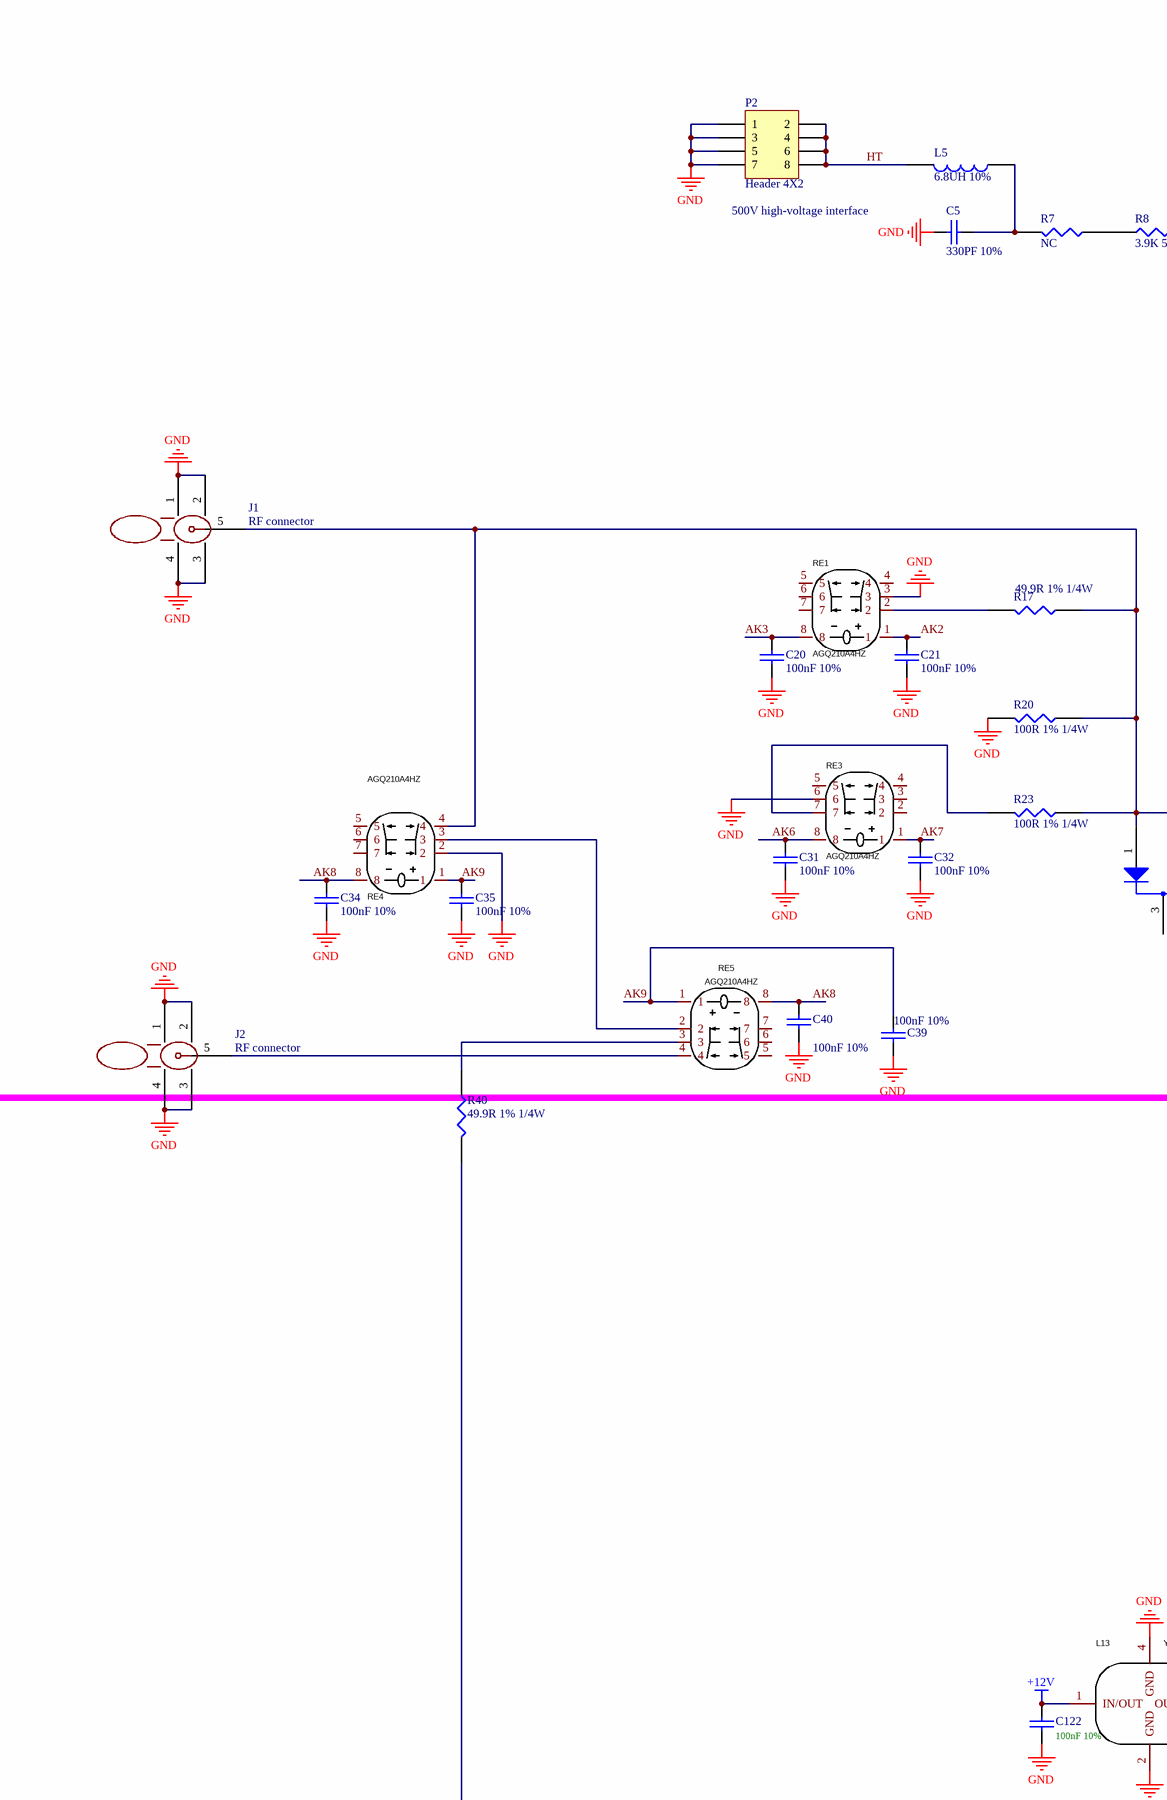
[diagram p0: PCBE109560-3.SchDoc, top left]
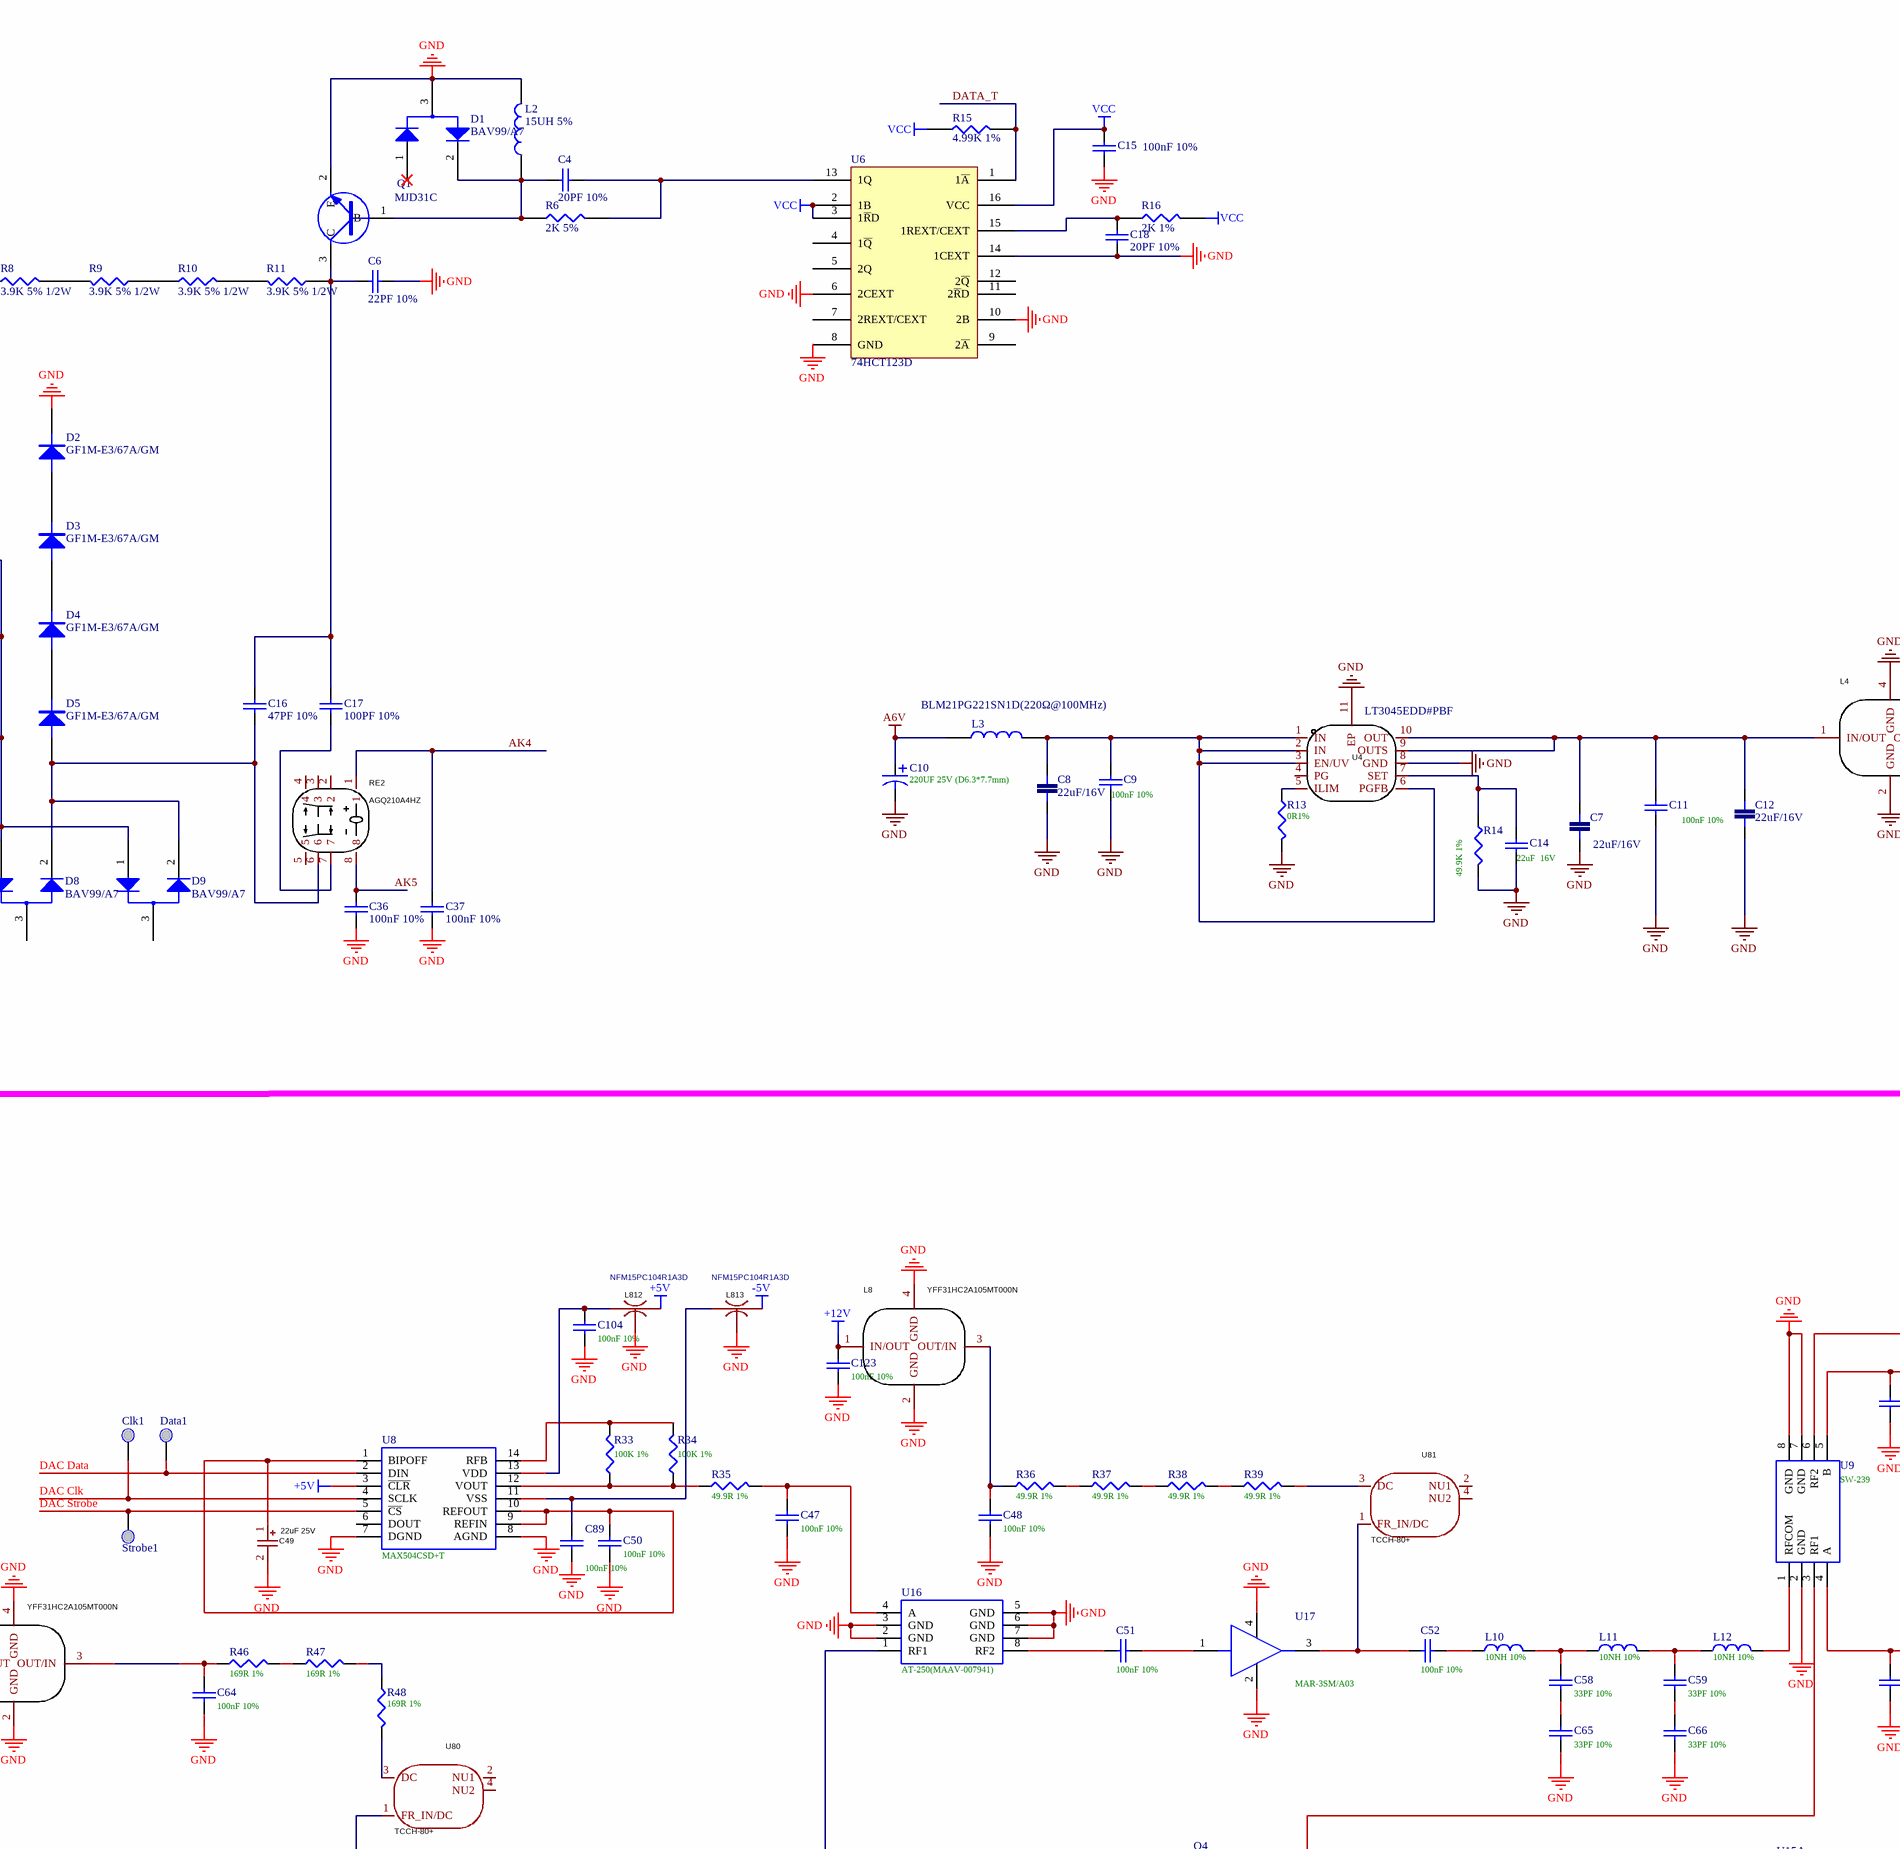
[diagram p1: PCBE109560-3.SchDoc, top middle]
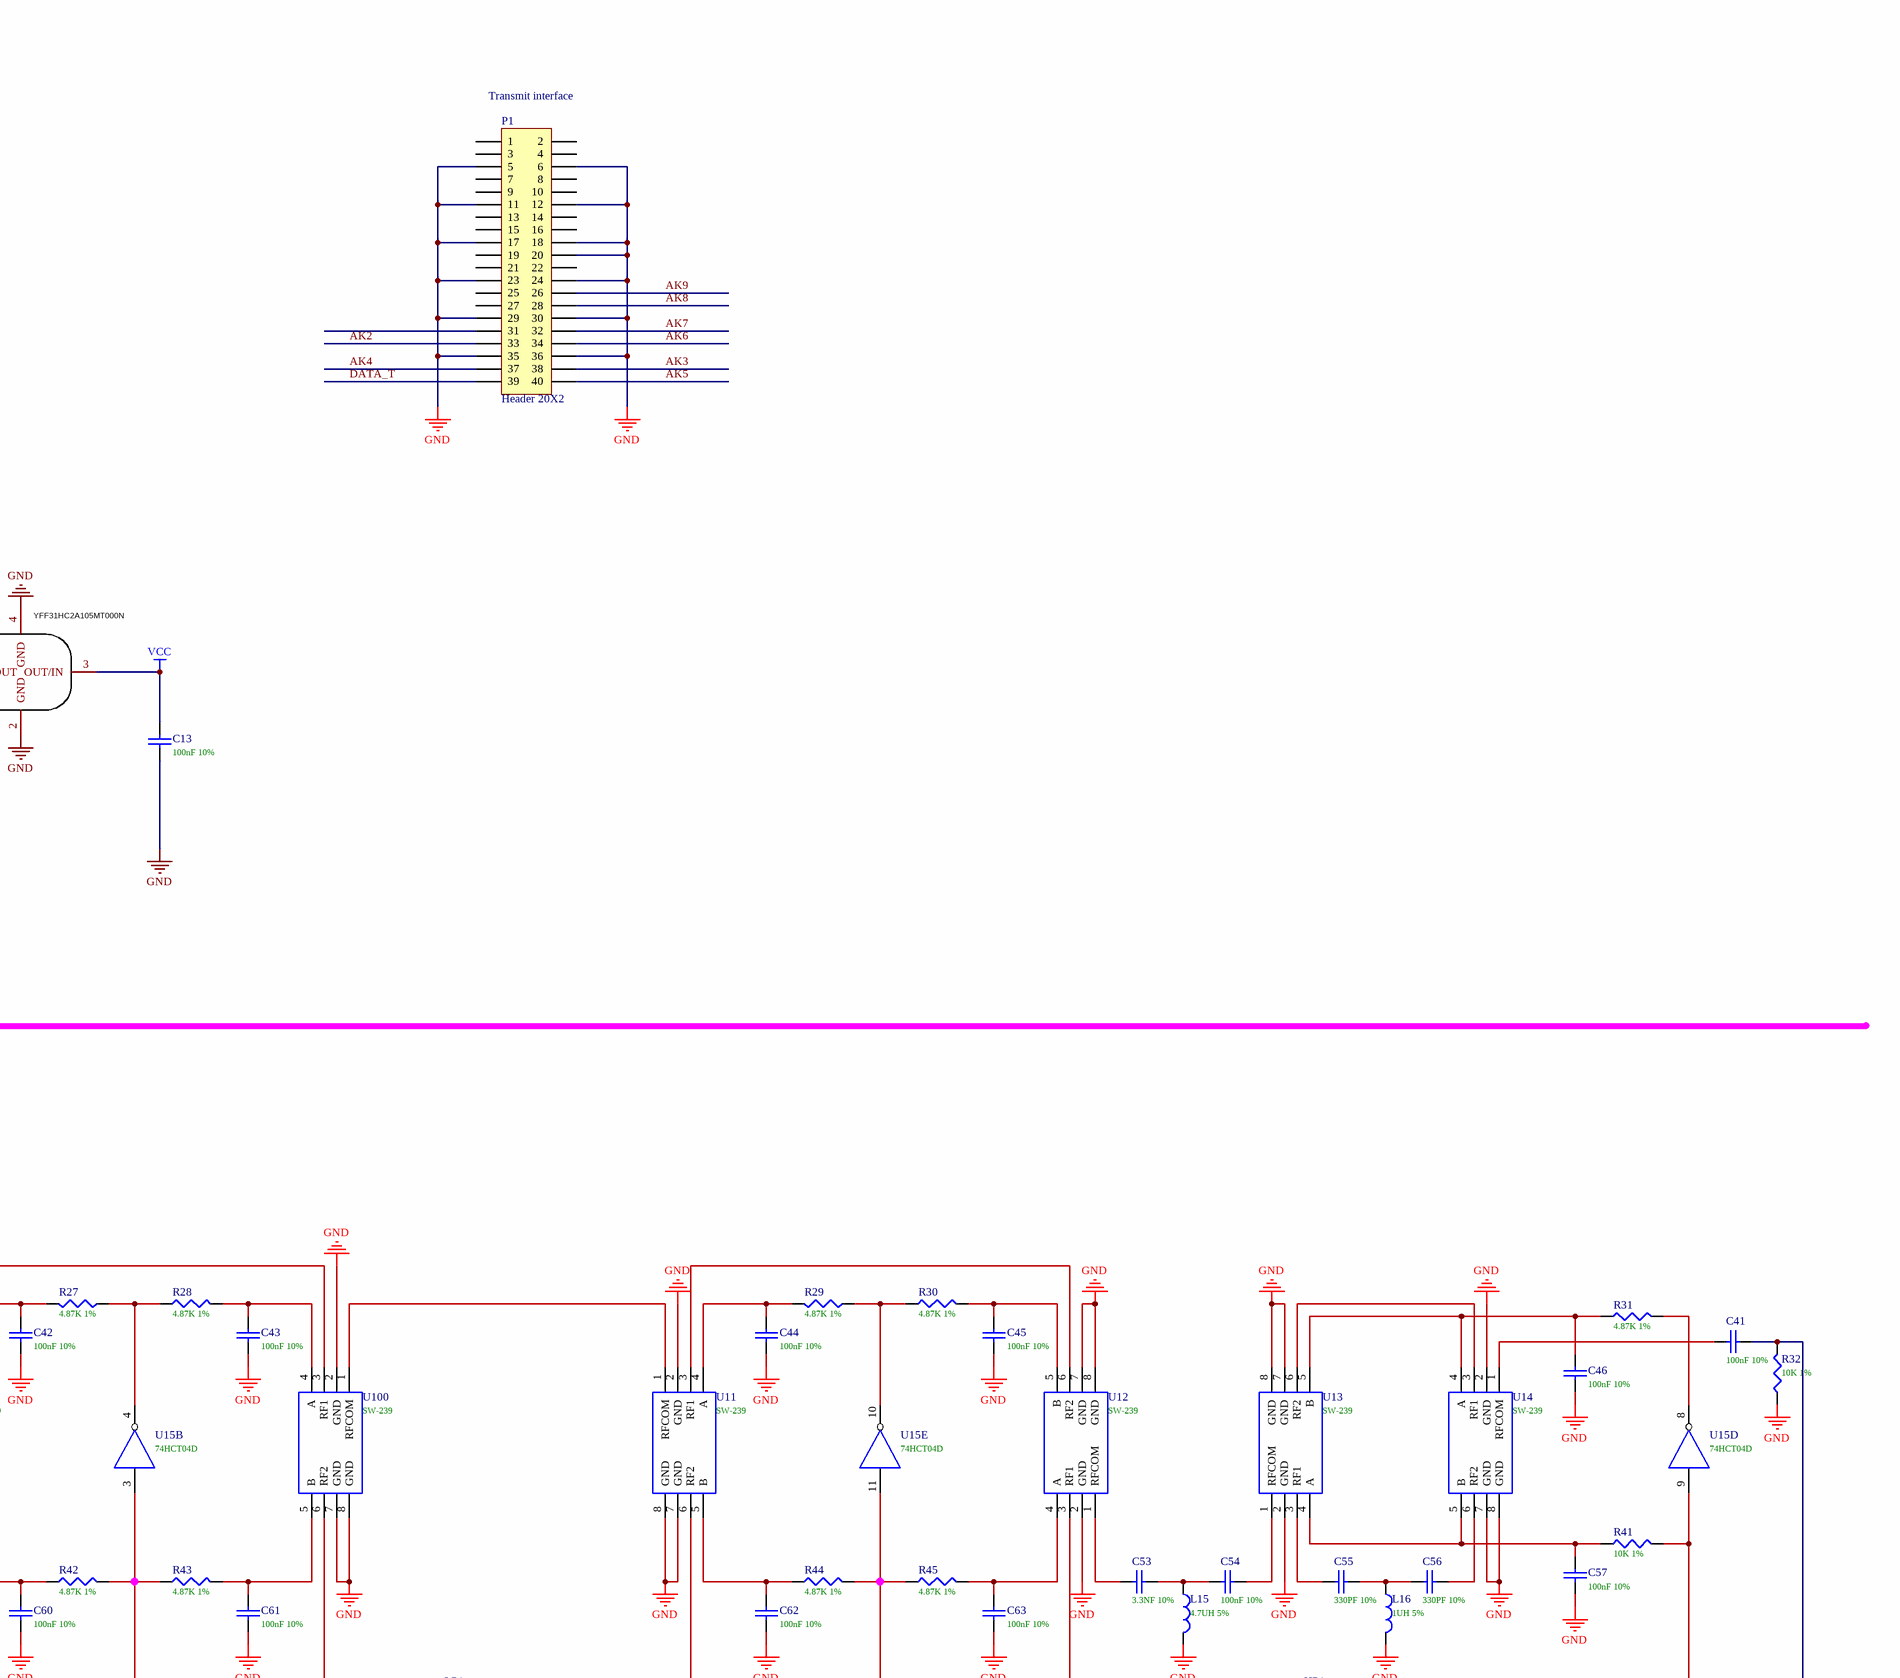
[diagram p2: PCBE109560-3.SchDoc, top right]
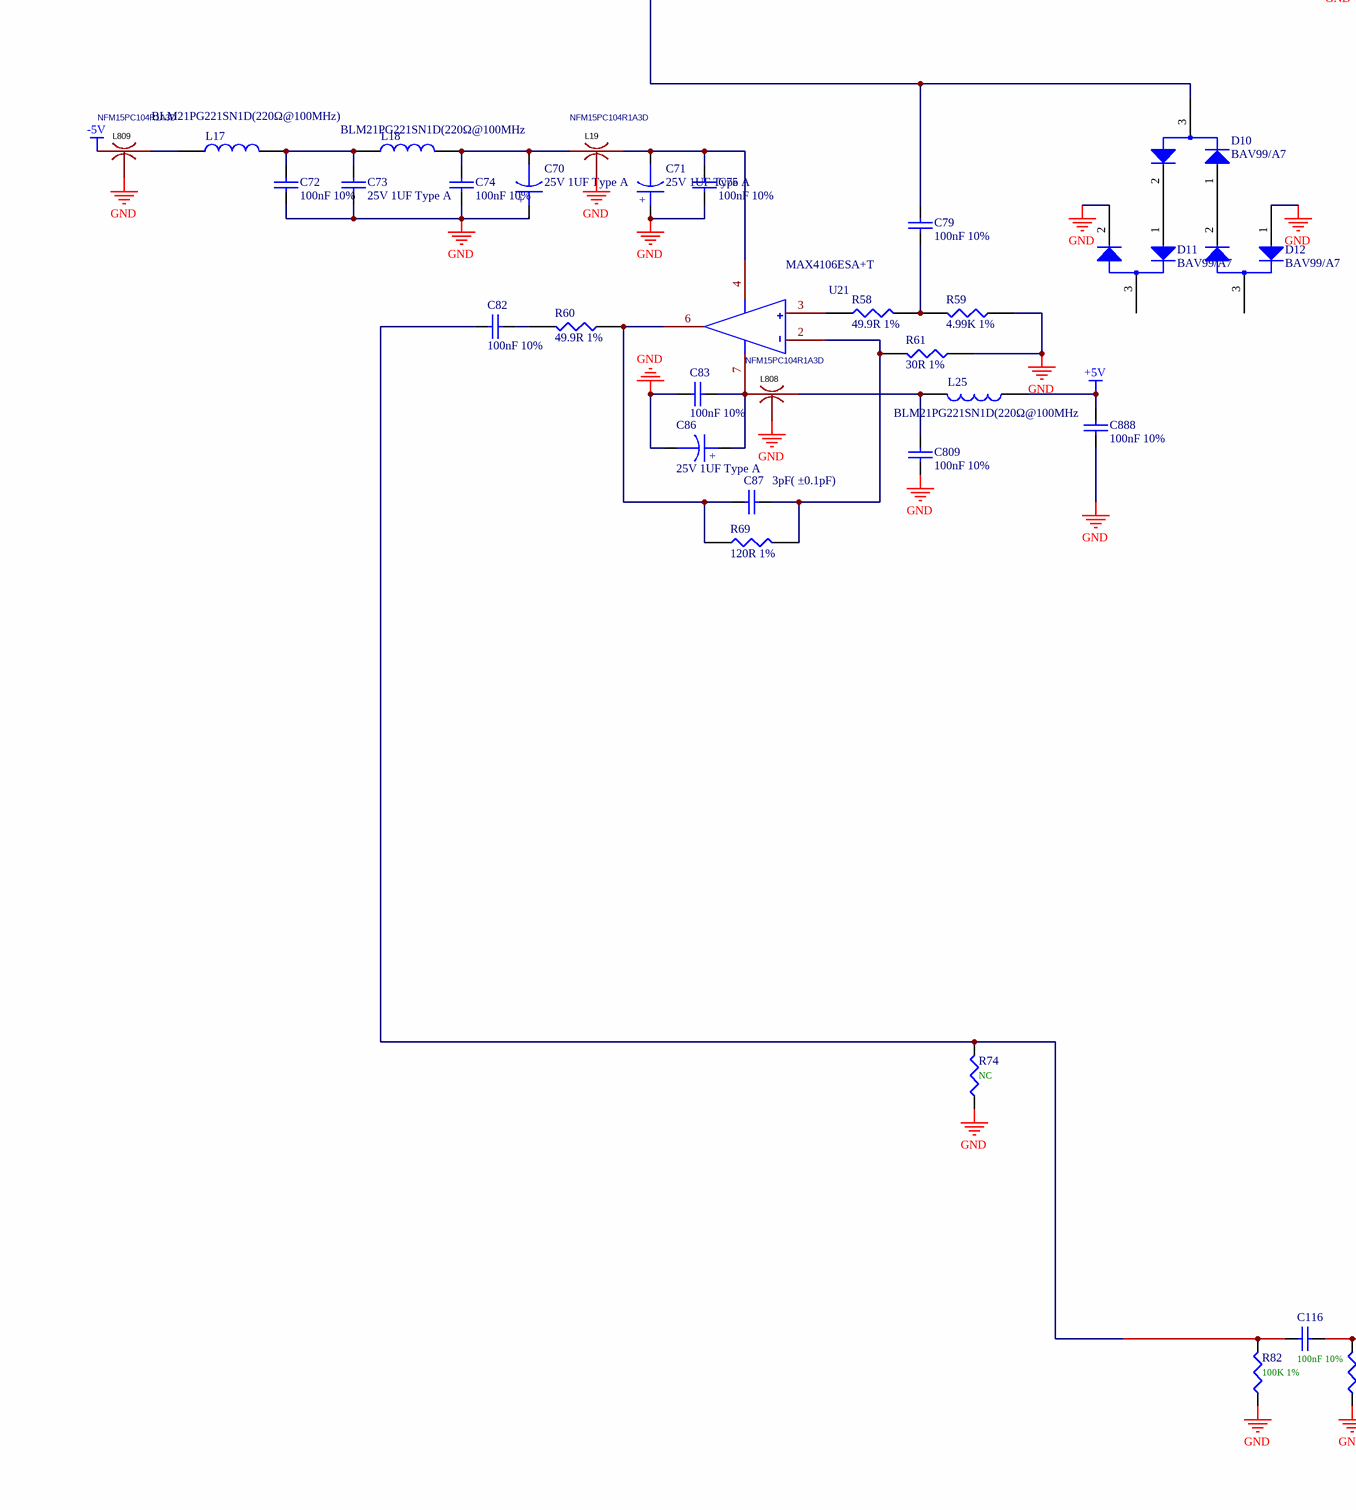
[diagram p3: PCBE109560-3.SchDoc, bottom left]
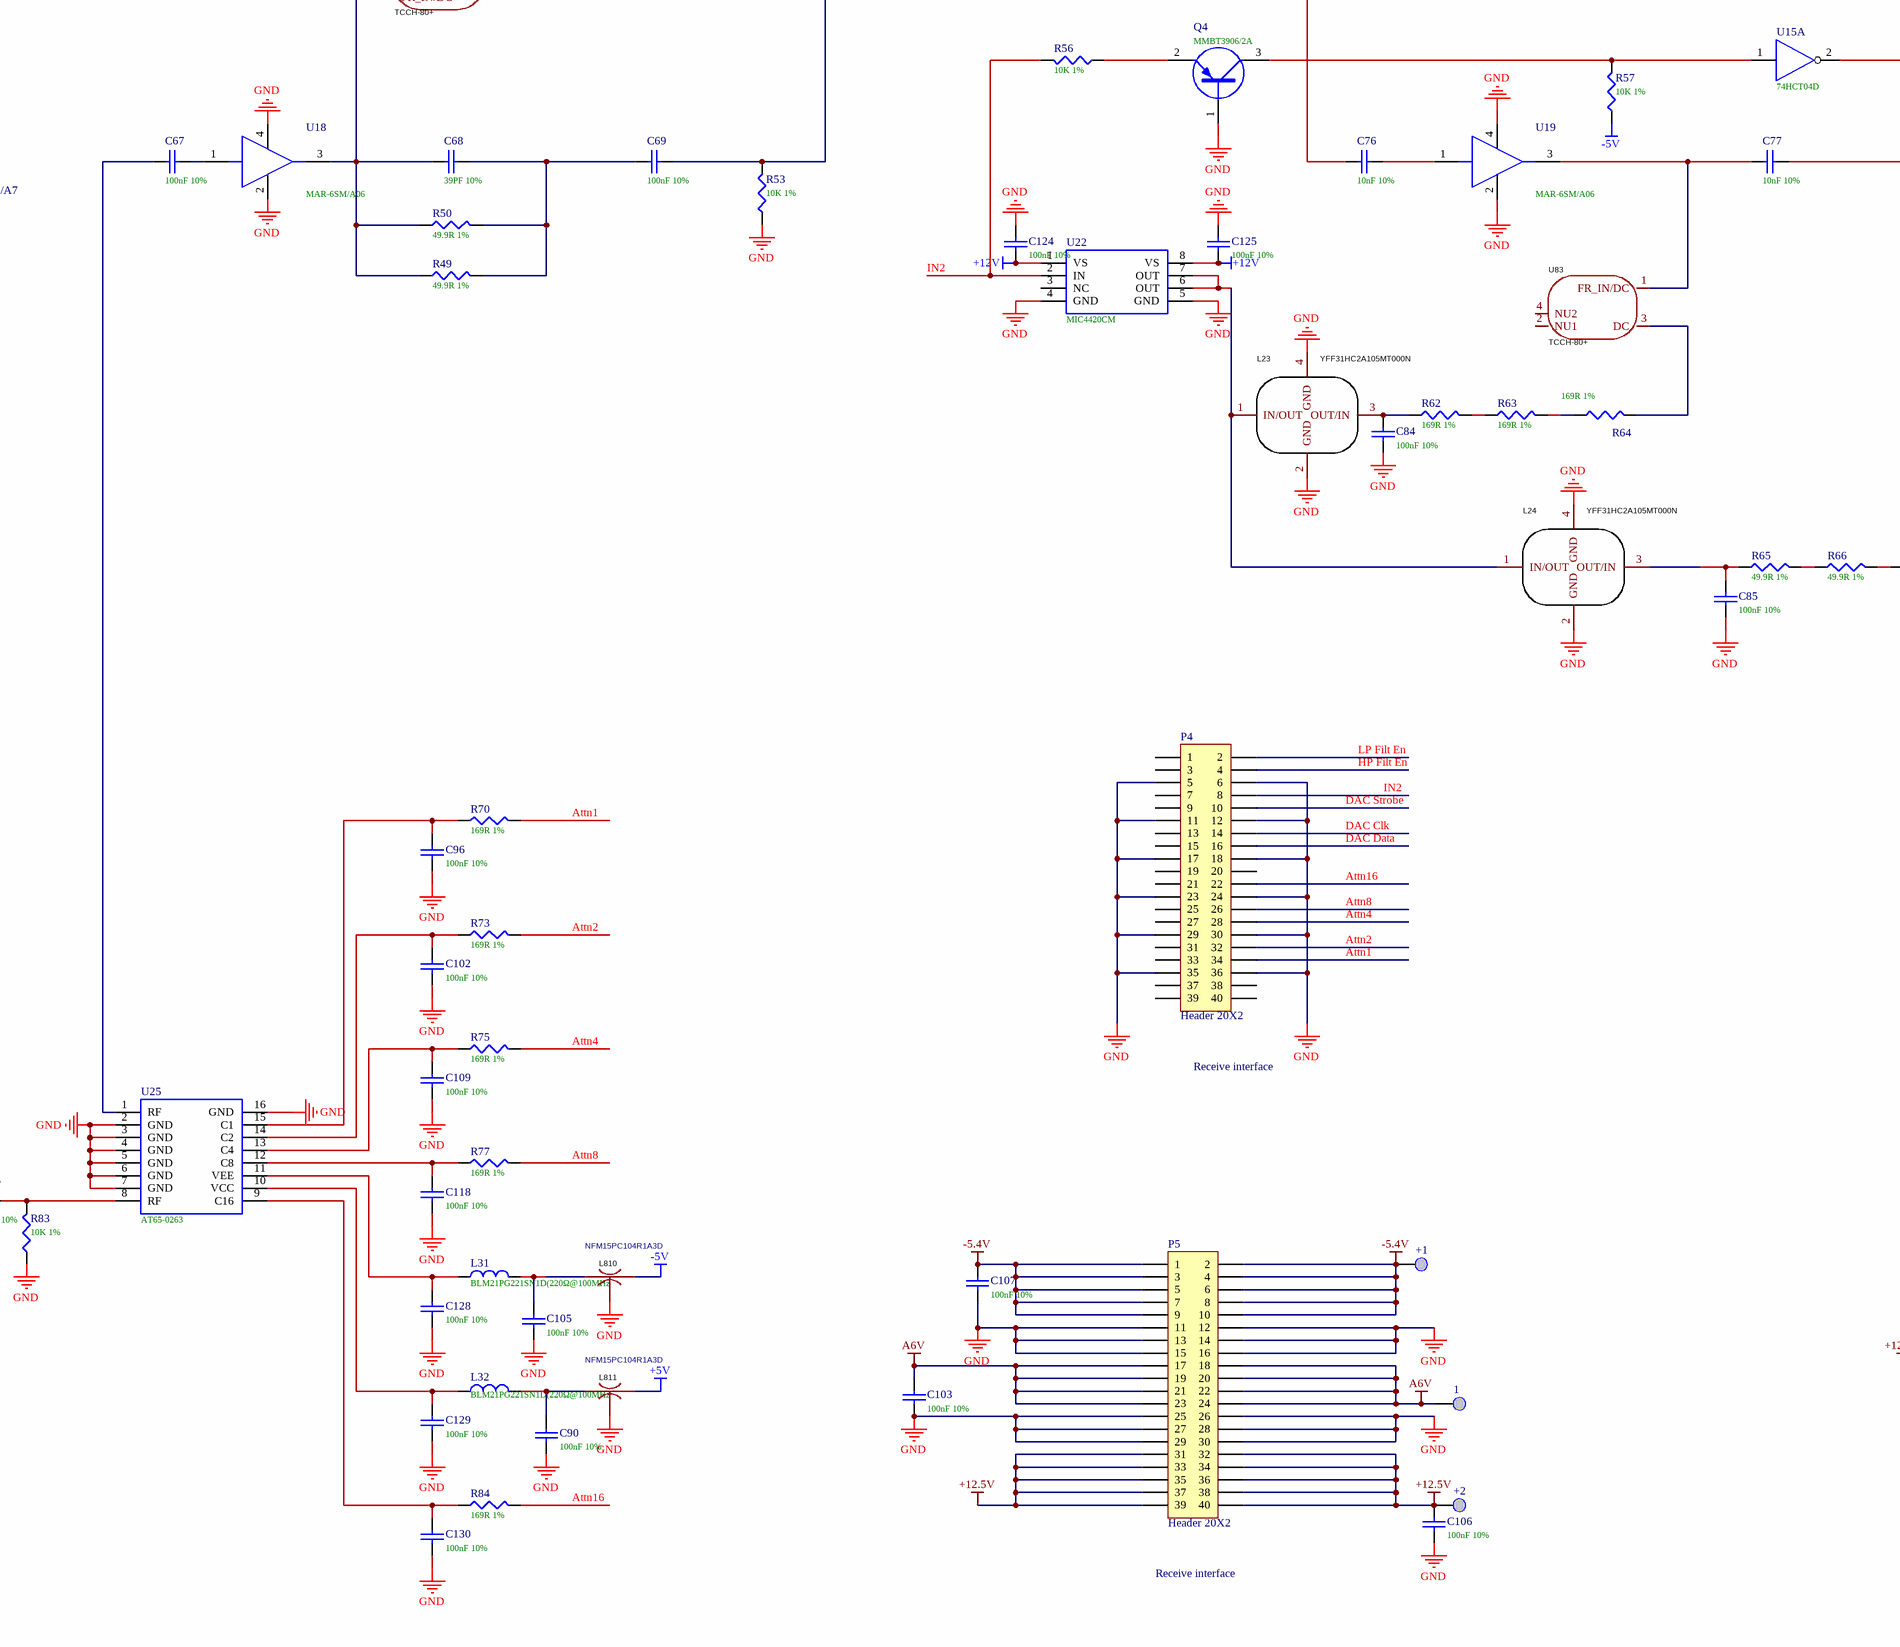
[diagram p4: PCBE109560-3.SchDoc, bottom middle]
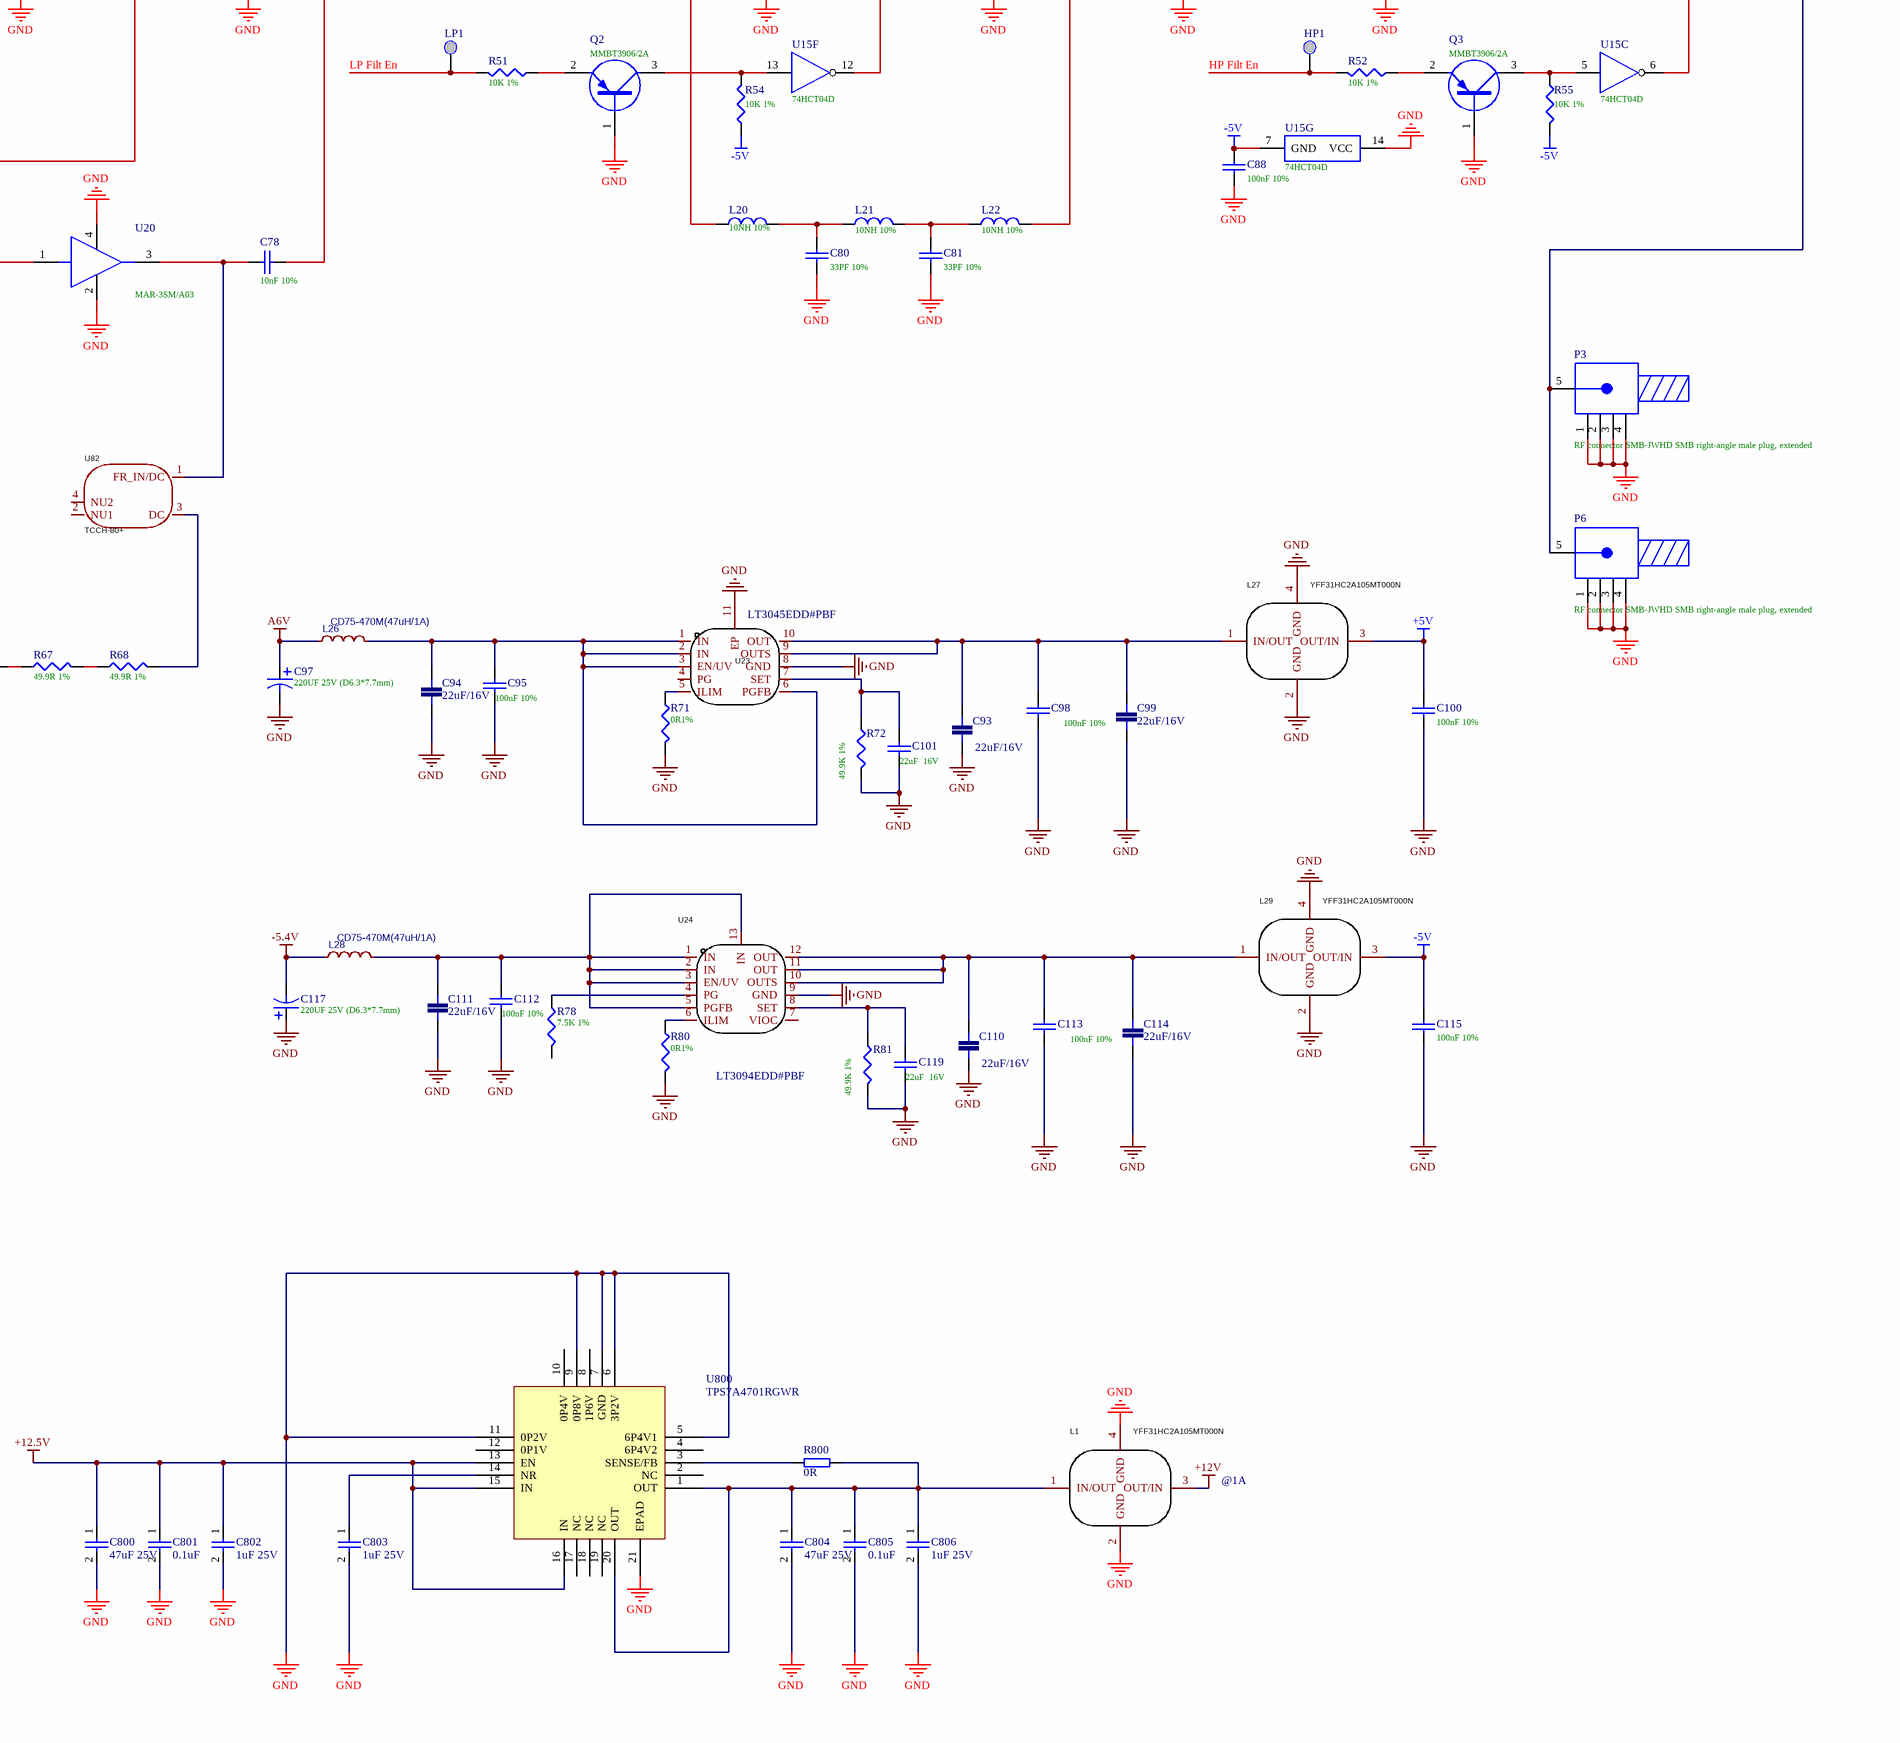
[diagram p5: PCBE109560-3.SchDoc, bottom right]
# Altium schematic sheet PCBE109560-3.SchDoc (part 1 of 2)
size E; SheetNumber: 0; SheetTotal: 0